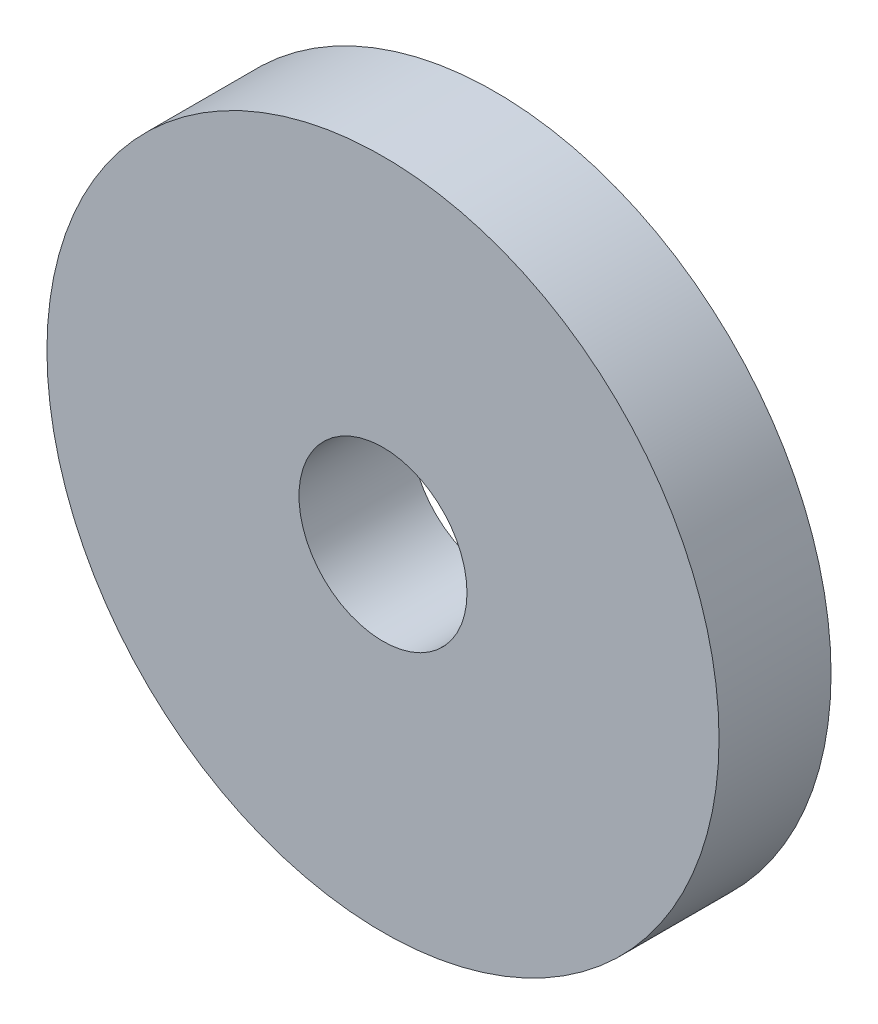
from build123d import *

# Parameters (mm, degrees)
SKETCH_1_R      = 60
SKETCH_1_R_2    = 15
EXTRUDE_1_DEPTH = 10


with BuildPart() as part:
    # 草图1 → 凸台-拉伸1 (new, symmetric)
    with BuildSketch(Plane.XY):
        Circle(SKETCH_1_R)
        Circle(SKETCH_1_R_2, mode=Mode.SUBTRACT)
    extrude(amount=EXTRUDE_1_DEPTH, both=True)


solid = part.part
